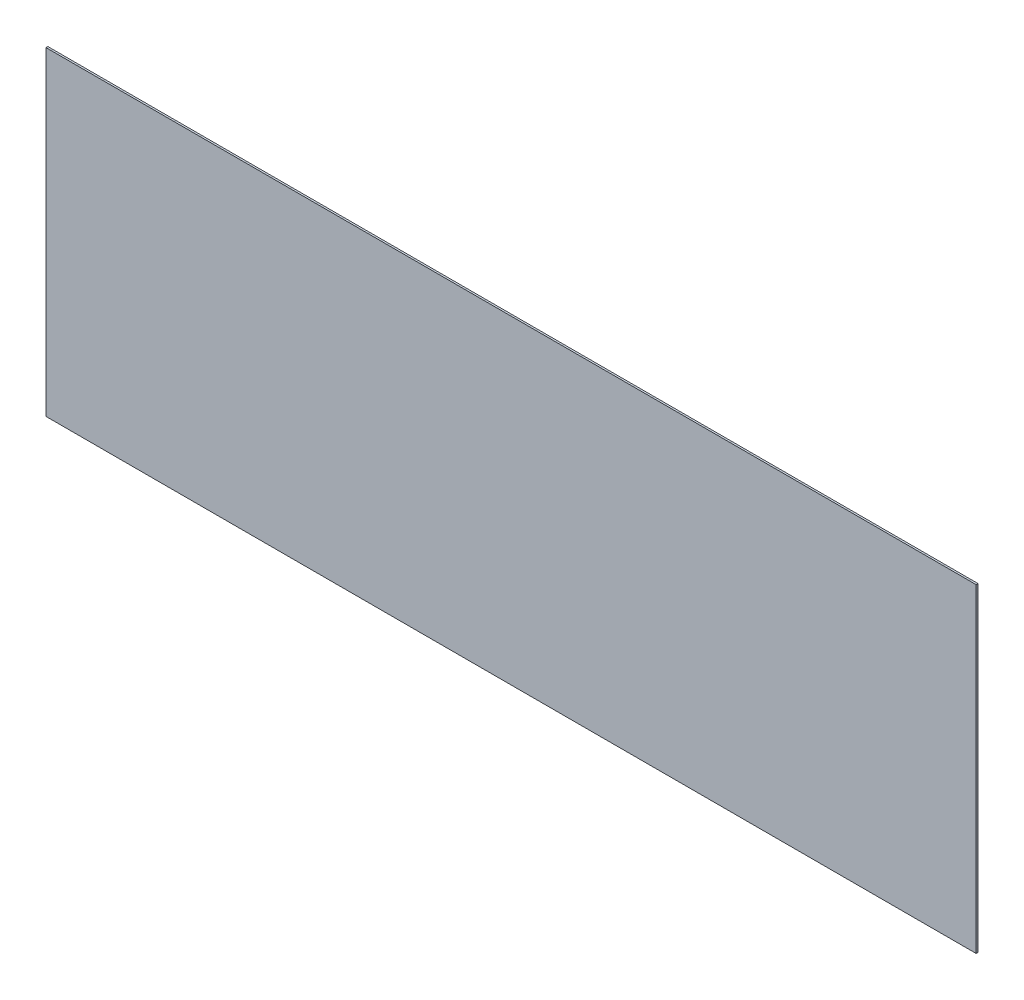
SolidWorks part; units mm, degrees
ref_plane "前视基准面" through (0, 0, 0) normal (0, 0, 1) x (1, 0, 0)
ref_plane "上视基准面" through (0, 0, 0) normal (0, 1, 0) x (1, 0, 0)
ref_plane "右视基准面" through (0, 0, 0) normal (1, 0, 0) x (0, 0, -1)
sketch "草图1" plane through (0, 0, 0) normal (0, 0, 1) x (1, 0, 0)
  line L1 (-286.5035, 182.4825) -> (703.4965, 182.4825)
  line L2 (-286.5035, 182.4825) -> (-286.5035, -157.5175)
  line L3 (-286.5035, -157.5175) -> (703.4965, -157.5175)
  line L4 (703.4965, 182.4825) -> (703.4965, -157.5175)
  dimension "D1" = 340
  dimension "D2" = 990
extrude "凸台-拉伸1" add sketch "草图1" along normal blind 2
